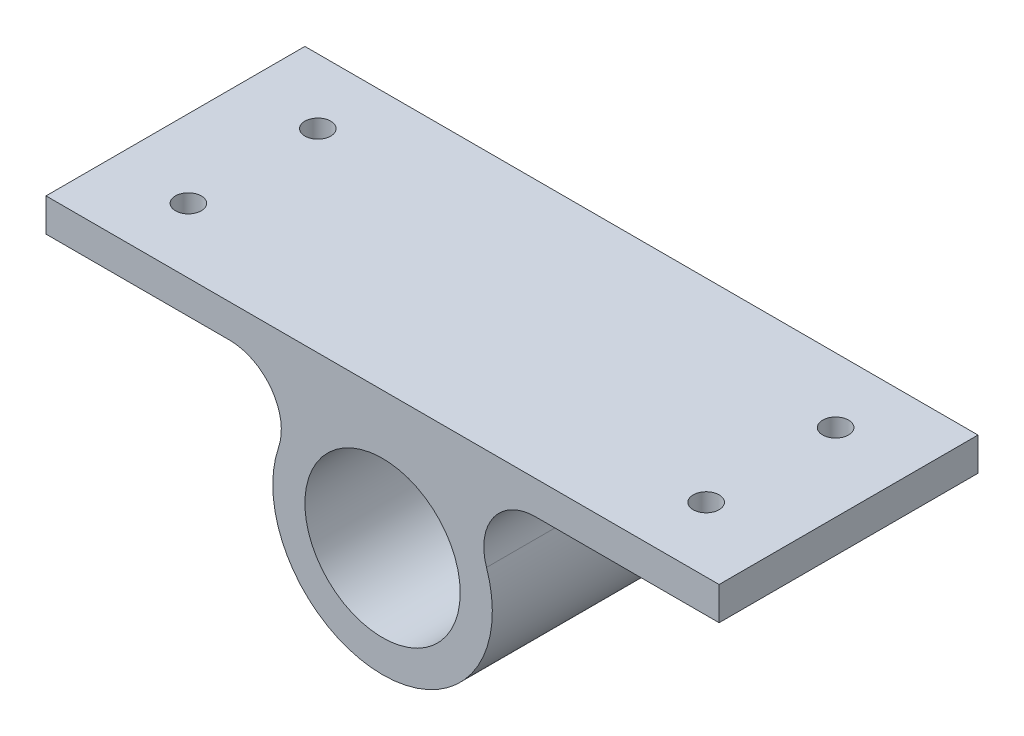
from build123d import *

# Parameters (mm, degrees)
SKETCH1_R           = 75
BOSS_EXTRUDE1_DEPTH = 250
CUT_EXTRUDE1_REACH  = 476.098
SKETCH2_R           = 12.5


with BuildPart() as part:
    # Sketch1 → Boss-Extrude1 (new body)
    with BuildSketch(Plane.XY):
        with BuildLine():
            Line((325, 132), (-325, 132))
            Line((-325, 132), (-325, 100))
            Line((-325, 100), (-147.770091697, 100))
            ThreePointArc((-147.770091697, 100), (-107.142009959, 79.143763902), (-100.407882819, 33.974358974))
            ThreePointArc((-100.407882819, 33.974358974), (0, -106), (100.407882819, 33.974358974))
            ThreePointArc((100.407882819, 33.974358974), (107.142009959, 79.143763902), (147.770091697, 100))
            Line((147.770091697, 100), (325, 100))
            Line((325, 100), (325, 132))
        make_face()
        Circle(SKETCH1_R, mode=Mode.SUBTRACT)
    extrude(amount=BOSS_EXTRUDE1_DEPTH)

    # Sketch2 → Cut-Extrude1 (cut, up to next)
    with BuildSketch(Plane(origin=(0, 132, 0), x_dir=(1, 0, 0), z_dir=(0, 1, 0)), mode=Mode.PRIVATE) as cut_extrude1_sk1:
        with Locations(Location((-250, -62.5, 0), (0, 0, 270))):
            Circle(SKETCH2_R)
    cut_extrude1_tool1 = extrude(cut_extrude1_sk1.sketch, amount=-CUT_EXTRUDE1_REACH, mode=Mode.PRIVATE) & part.part
    # Sketch2 → Cut-Extrude1 (cut, up to next)
    with BuildSketch(Plane(origin=(0, 132, 0), x_dir=(1, 0, 0), z_dir=(0, 1, 0)), mode=Mode.PRIVATE) as cut_extrude1_sk2:
        with Locations(Location((-250, -187.5, 0), (0, 0, 270))):
            Circle(SKETCH2_R)
    cut_extrude1_tool2 = extrude(cut_extrude1_sk2.sketch, amount=-CUT_EXTRUDE1_REACH, mode=Mode.PRIVATE) & part.part
    # Sketch2 → Cut-Extrude1 (cut, up to next)
    with BuildSketch(Plane(origin=(0, 132, 0), x_dir=(1, 0, 0), z_dir=(0, 1, 0)), mode=Mode.PRIVATE) as cut_extrude1_sk3:
        with Locations(Location((250, -187.5, 0), (0, 0, 270))):
            Circle(SKETCH2_R)
    cut_extrude1_tool3 = extrude(cut_extrude1_sk3.sketch, amount=-CUT_EXTRUDE1_REACH, mode=Mode.PRIVATE) & part.part
    # Sketch2 → Cut-Extrude1 (cut, up to next)
    with BuildSketch(Plane(origin=(0, 132, 0), x_dir=(1, 0, 0), z_dir=(0, 1, 0)), mode=Mode.PRIVATE) as cut_extrude1_sk4:
        with Locations(Location((250, -62.5, 0), (0, 0, 270))):
            Circle(SKETCH2_R)
    cut_extrude1_tool4 = extrude(cut_extrude1_sk4.sketch, amount=-CUT_EXTRUDE1_REACH, mode=Mode.PRIVATE) & part.part
    add(cut_extrude1_tool1.solids().sort_by_distance((-250, 132, 62.5))[0], mode=Mode.SUBTRACT)
    add(cut_extrude1_tool2.solids().sort_by_distance((-250, 132, 187.5))[0], mode=Mode.SUBTRACT)
    add(cut_extrude1_tool3.solids().sort_by_distance((250, 132, 187.5))[0], mode=Mode.SUBTRACT)
    add(cut_extrude1_tool4.solids().sort_by_distance((250, 132, 62.5))[0], mode=Mode.SUBTRACT)


solid = part.part
